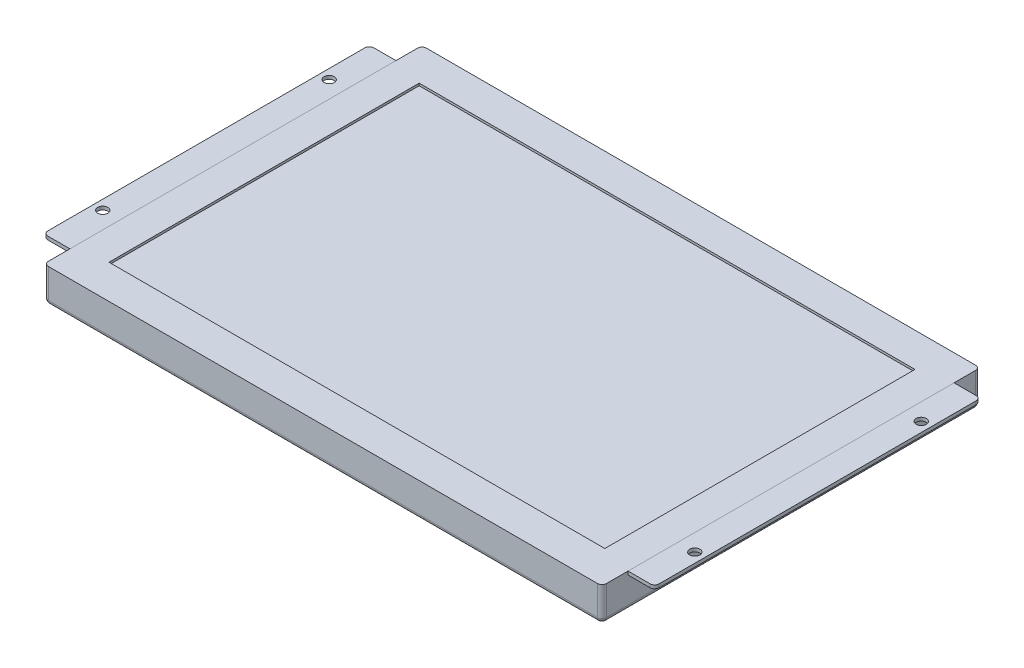
SolidWorks part; units mm, degrees
ref_plane "前视基准面" through (0, 0, 0) normal (0, 0, 1) x (1, 0, 0)
ref_plane "上视基准面" through (0, 0, 0) normal (0, 1, 0) x (1, 0, 0)
ref_plane "右视基准面" through (0, 0, 0) normal (1, 0, 0) x (0, 0, -1)
sketch "草图1" plane through (0, 0, 0) normal (0, 1, 0) x (1, 0, 0)
  line L1 (-123.25, 83.5) -> (123.25, 83.5)
  line L2 (-123.25, 83.5) -> (-123.25, -83.5)
  line L3 (-123.25, -83.5) -> (123.25, -83.5)
  line L4 (123.25, 83.5) -> (123.25, -83.5)
  line L5 (-123.25, 83.5) -> (123.25, -83.5) construction
  line L6 (-123.25, -83.5) -> (123.25, 83.5) construction
  point P0 (0, 0)
  dimension "D1" = 167
  dimension "D2" = 246.5
extrude "凸台-拉伸1" add sketch "草图1" along normal blind 15
sketch "草图3" plane through (0, 0, 0) normal (0, -1, 0) x (1, 0, 0)
  line L1 (80, -47) -> (-80, -47)
  line L2 (80, -47) -> (80, 47)
  line L3 (80, 47) -> (-80, 47)
  line L4 (-80, -47) -> (-80, 47)
  line L5 (80, -47) -> (-80, 47) construction
  line L6 (80, 47) -> (-80, -47) construction
  point P0 (0, 0)
  dimension "D1" = 160
  dimension "D2" = 94
extrude "凸台-拉伸2" add sketch "草图3" along normal blind 20
fillet "圆角1" radius 2 20 edges at (0, 0, -47) (80, 0, 0) (0, 0, 47) (-80, 0, 0) (0, 0, -83.5) (-123.25, 0, 0) (0, 0, 83.5) (123.25, 0, 0) (0, -20, 47) (80, -20, 0) (0, -20, -47) (-80, -20, 0) (-123.25, 7.5, 83.5) (123.25, 7.5, 83.5) (123.25, 7.5, -83.5) (-123.25, 7.5, -83.5) (-80, -10, 47) (-80, -10, -47) (80, -10, 47) (80, -10, -47)
sketch "草图4" plane through (0, 15, 0) normal (0, 1, 0) x (1, 0, 0)
  line L1 (-109.5, 68.5) -> (109.5, 68.5)
  line L2 (-109.5, 68.5) -> (-109.5, -68.5)
  line L3 (-109.5, -68.5) -> (109.5, -68.5)
  line L4 (109.5, 68.5) -> (109.5, -68.5)
  line L5 (-109.5, 68.5) -> (109.5, -68.5) construction
  line L6 (-109.5, -68.5) -> (109.5, 68.5) construction
  point P0 (0, 0)
  dimension "D1" = 219
  dimension "D2" = 137
extrude "切除-拉伸1" cut sketch "草图4" against normal blind 1
sketch "草图5" plane through (0, 15, 0) normal (0, 1, 0) x (1, 0, 0)
  line L0 (0, 0) -> (164.8443, 0) construction
  line L1 (123.25, -81.5) -> (123.25, 81.5) construction
  line L2 (135, -72) -> (123.25, -72)
  line L3 (135, -72) -> (135, 72)
  line L4 (135, 72) -> (123.25, 72)
  line L5 (123.25, -72) -> (123.25, 72)
  line L6 (135, -72) -> (123.25, 72) construction
  line L7 (135, 72) -> (123.25, -72) construction
  line L8 (0, 0) -> (0, 46.0219) construction
  line L9 (-135, 72) -> (-123.25, -72) construction
  line L10 (-135, -72) -> (-123.25, 72) construction
  line L11 (-123.25, -72) -> (-123.25, 72)
  line L12 (-135, 72) -> (-123.25, 72)
  line L13 (-135, -72) -> (-135, 72)
  line L14 (-135, -72) -> (-123.25, -72)
  point P3 (129.125, 0)
  point P15 (-129.125, 0)
  dimension "D1" = 270
  dimension "D2" = 144
extrude "凸台-拉伸3" add sketch "草图5" against normal blind 1.5 separate body
hole_wizard "Ø4.5 (4.5) 直径孔1" positions "草图7" profile "草图6" hole size "Ø4.5" standard "GB" end condition through all
sketch "草图7" plane through (0, 15, 0) normal (0, 1, 0) x (1, 0, 0)
  line L0 (0, 0) -> (178.02, 0) construction
  line L3 (0, 0) -> (0, 47.1394) construction
  point P0 (130.75, 50)
  point P2 (130.75, -50)
  point P20 (-130.75, -50)
  point P21 (-130.75, 50)
  dimension "D1" = 100
  dimension "D2" = 261.5
sketch "草图6" plane through (130.75, 15, -50) normal (1, 0, 0) x (0, 0, 1)
  line L0 (0, 0) -> (0, 35)
  line L1 (0, 35) -> (2.25, 35)
  line L2 (2.25, 35) -> (2.25, 0)
  line L5 (2.25, 0) -> (0, 0)
  line L11 (0, -6.35) -> (0, 107.95) construction
  dimension "通孔孔直径" = 4.5
  dimension "通孔孔深度" = 35
fillet "圆角2" radius 2 2 edges at (135, 14.25, 72) (135, 14.25, -72)
fillet "圆角3" radius 2 2 edges at (-135, 14.25, 72) (-135, 14.25, -72)
